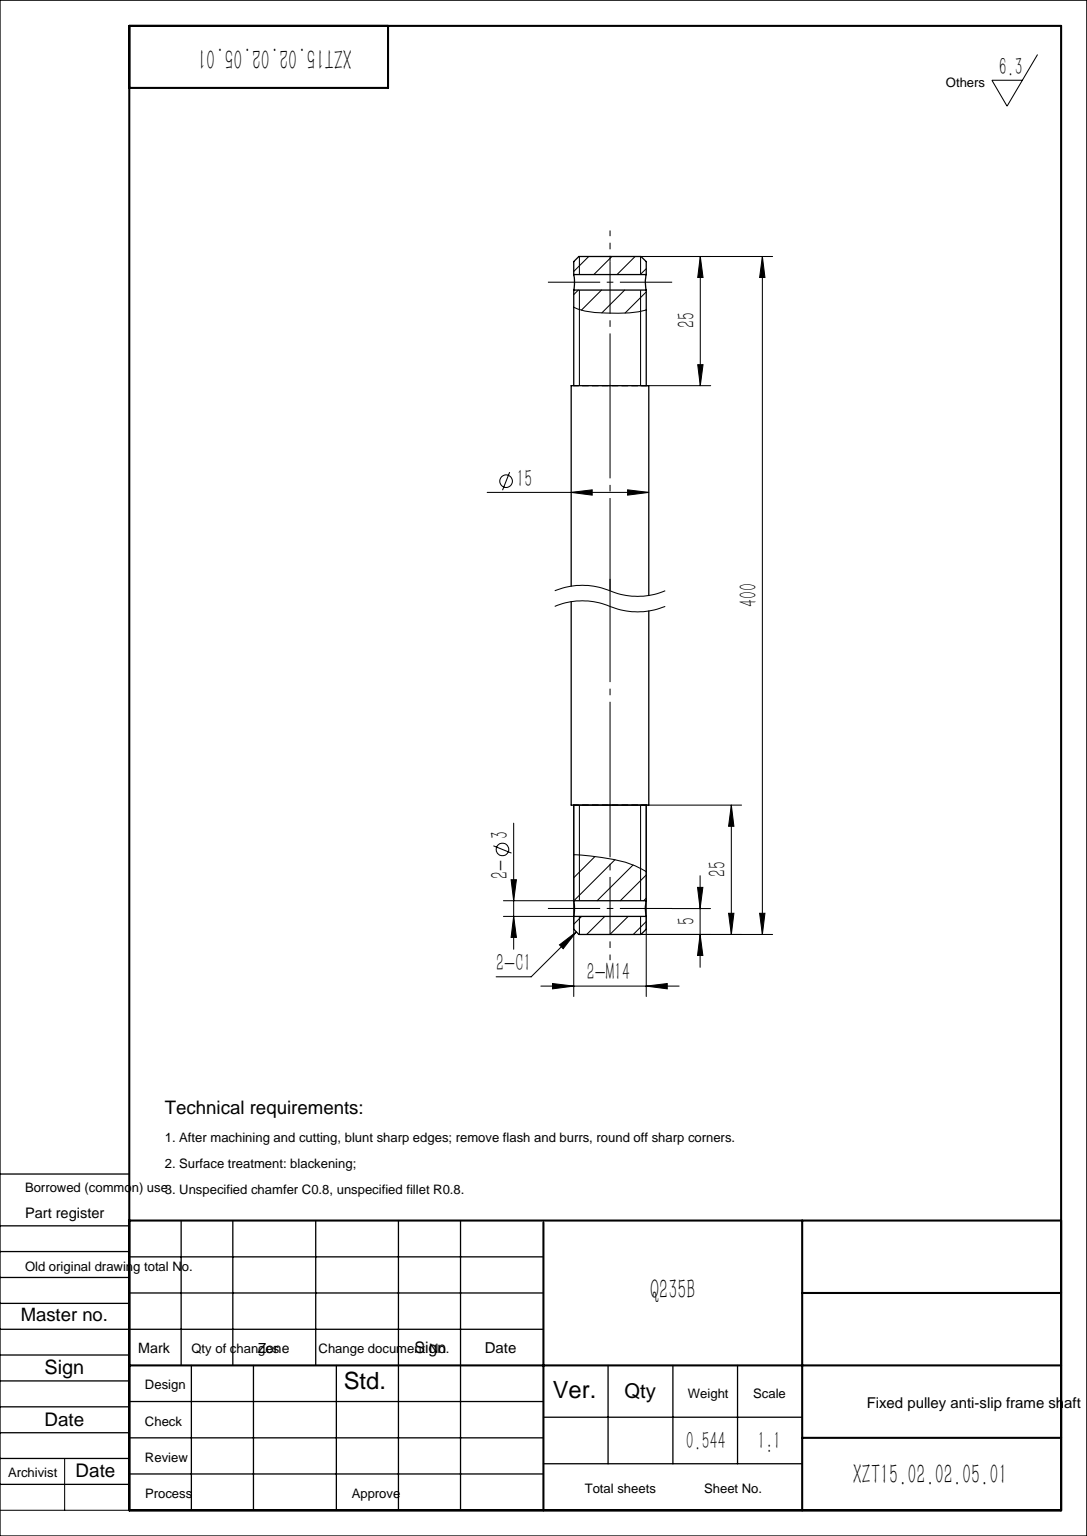
SolidWorks part; units mm, degrees
material "Q235B"
ref_plane "Front Plane" through (0, 0, 0) normal (0, 0, 1) x (1, 0, 0)
ref_plane "Top Plane" through (0, 0, 0) normal (0, 1, 0) x (1, 0, 0)
ref_plane "Right Plane" through (0, 0, 0) normal (1, 0, 0) x (0, 0, -1)
sketch "Sketch1" plane through (0, 0, 0) normal (0, 0, 1) x (1, 0, 0)
  line L0 (0, 0) -> (7, 0)
  line L1 (7, 0) -> (7, 25)
  line L2 (7, 25) -> (7.5, 25)
  line L3 (7.5, 25) -> (7.5, 375)
  line L4 (7.5, 375) -> (7, 375)
  line L5 (7, 375) -> (7, 400)
  line L6 (7, 400) -> (0, 400)
  line L7 (0, 400) -> (0, 0)
  line L8 (0, 0) -> (0, -3.5159) construction
  dimension "D1" = 14
  dimension "D2" = 15
  dimension "D3" = 400
  dimension "D4" = 25
revolve "Revolve1" add sketch "Sketch1" angle 360 about L8
cosmetic thread "Cosmetic Thread1"
cosmetic thread "Cosmetic Thread2"
chamfer "Chamfer1" distance 1 angle 45 2 edges at (0, 0, 7) (0, 400, 7)
sketch "Sketch3" plane through (0, 0, 0) normal (1, 0, 0) x (0, 0, -1)
  line L0 (0, 400) -> (0, 395) construction
  line L1 (6, 400) -> (-6, 400) construction
  line L2 (7.5, 200) -> (58.4347, 200) construction
  line L3 (7.5, 25) -> (7.5, 375) construction
  line L4 (0, 0) -> (0, 5) construction
  circle A0 centre (0, 395) radius 1.5
  circle A1 centre (0, 5) radius 1.5
  dimension "D2" = 3
  dimension "D1" = 5
extrude "Cut-Extrude1" cut sketch "Sketch3" against normal through all both and the other way through all
